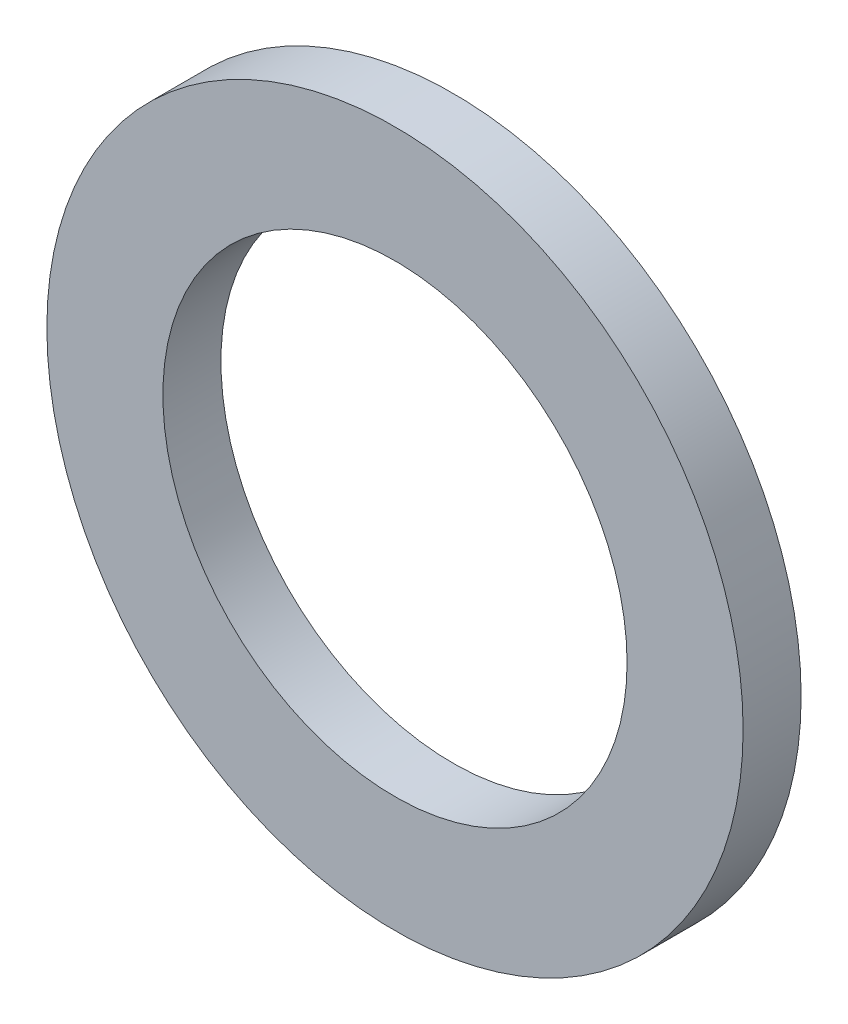
from build123d import *

# Parameters (mm, degrees)
SKETCH1_R           = 60
SKETCH1_R_2         = 40
BOSS_EXTRUDE1_DEPTH = 10


with BuildPart() as part:
    # Sketch1 → Boss-Extrude1 (new body)
    with BuildSketch(Plane.XY):
        Circle(SKETCH1_R)
        Circle(SKETCH1_R_2, mode=Mode.SUBTRACT)
    extrude(amount=BOSS_EXTRUDE1_DEPTH)


solid = part.part
